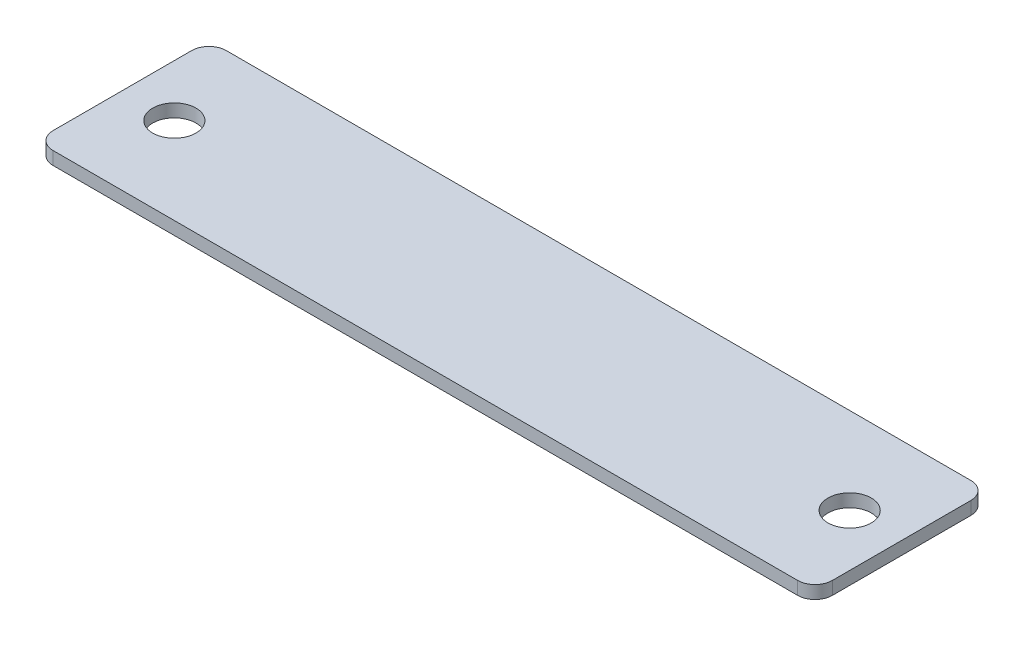
SolidWorks part; units mm, degrees
material "Q235"
ref_plane "前视基准面" through (0, 0, 0) normal (0, 0, 1) x (1, 0, 0)
ref_plane "上视基准面" through (0, 0, 0) normal (0, 1, 0) x (1, 0, 0)
ref_plane "右视基准面" through (0, 0, 0) normal (1, 0, 0) x (0, 0, -1)
sketch "草图1" plane through (0, 0, 0) normal (0, 1, 0) x (1, 0, 0)
  line L1 (-45, -10) -> (45, -10)
  line L2 (-45, -10) -> (-45, 10)
  line L3 (-45, 10) -> (45, 10)
  line L4 (45, -10) -> (45, 10)
  line L5 (-45, -10) -> (45, 10) construction
  line L6 (-45, 10) -> (45, -10) construction
  point P0 (0, 0)
  dimension "D1" = 20
  dimension "D2" = 90
extrude "凸台-拉伸1" add sketch "草图1" along normal blind 1.5
sketch "草图2" plane through (0, 1.5, 0) normal (0, 1, 0) x (1, 0, 0)
  line L0 (0, 10) -> (0, -10) construction
  line L1 (45, 10) -> (-45, 10) construction
  line L2 (-45, -10) -> (45, -10) construction
  line L3 (-45, 0) -> (45, 0) construction
  line L4 (-45, 10) -> (-45, -10) construction
  line L5 (45, -10) -> (45, 10) construction
  circle A0 centre (-39, 0) radius 2.5
  circle A1 centre (39, 0) radius 2.5
  dimension "D1" = 78
  dimension "D2" = 5
extrude "切除-拉伸1" cut sketch "草图2" against normal through all
fillet "圆角1" radius 2 4 edges at (45, 0.75, 10) (45, 0.75, -10) (-45, 0.75, 10) (-45, 0.75, -10)
